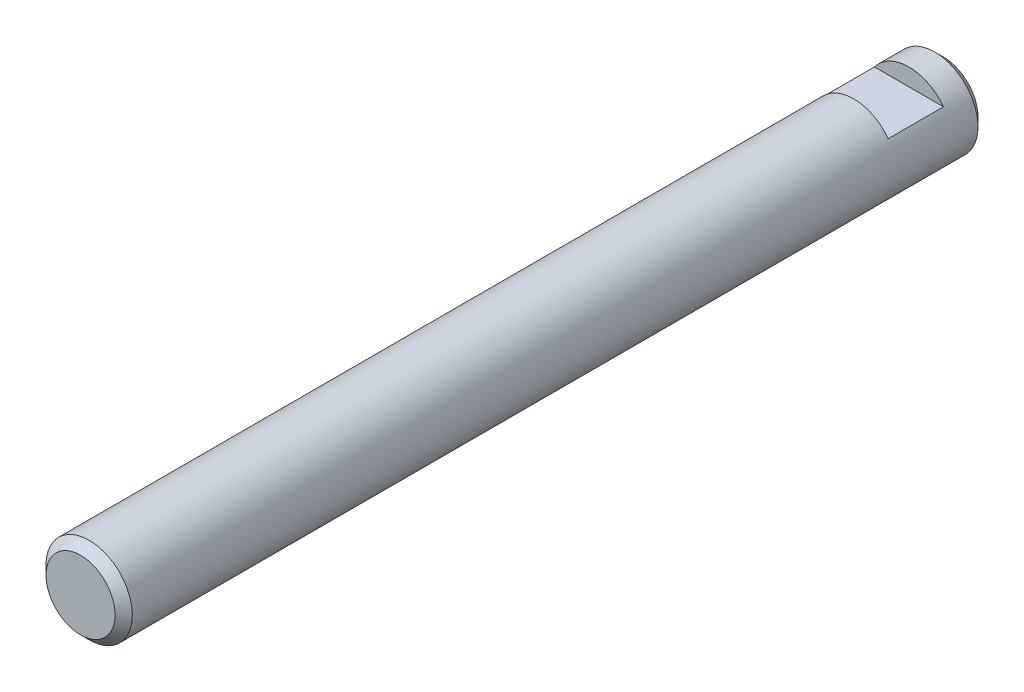
SolidWorks part; units mm, degrees
material "不锈钢 (铁素体)"
ref_plane "前视基准面" through (0, 0, 0) normal (0, 0, 1) x (1, 0, 0)
ref_plane "上视基准面" through (0, 0, 0) normal (0, 1, 0) x (1, 0, 0)
ref_plane "右视基准面" through (0, 0, 0) normal (1, 0, 0) x (0, 0, -1)
sketch "草图1" plane through (0, 0, 0) normal (0, 0, 1) x (1, 0, 0)
  circle A0 centre (0, 0) radius 2.5
  dimension "D1" = 5
extrude "凸台-拉伸1" add sketch "草图1" along normal mid plane 50
chamfer "倒角1" distance 0.5 angle 45 2 edges at (2.5, 0, -25) (2.5, 0, 25)
sketch "草图2" plane through (0, 0, 0) normal (1, 0, 0) x (0, 0, -1)
  line L0 (0, 0) -> (0, 6.0711) construction
  line L6 (19.8, 5.0251) -> (19.8, 1.5)
  line L7 (23, 1.5) -> (19.8, 1.5)
  line L8 (23, 5.0251) -> (23, 1.5)
  line L9 (23, 5.0251) -> (19.8, 5.0251)
  line L10 (25, -2) -> (25, 2) construction
  dimension "D1" = 3.2
  dimension "D2" = 2
extrude "切除-拉伸1" cut sketch "草图2" against normal through all both and the other way through all
